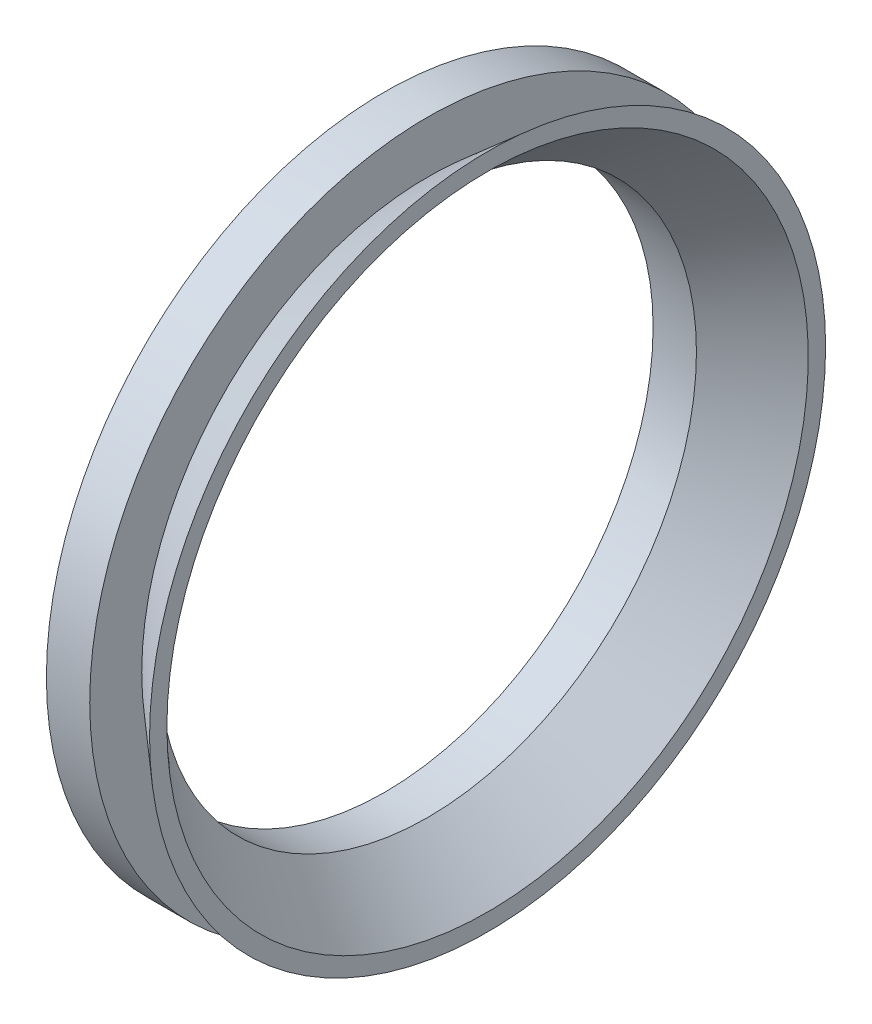
SolidWorks part; units mm, degrees
ref_plane "前视基准面" through (0, 0, 0) normal (0, 0, 1) x (1, 0, 0)
ref_plane "上视基准面" through (0, 0, 0) normal (0, 1, 0) x (1, 0, 0)
ref_plane "右视基准面" through (0, 0, 0) normal (1, 0, 0) x (0, 0, -1)
sketch "草图1" plane through (0, 0, 0) normal (0, 0, 1) x (1, 0, 0)
  line L0 (0, 0) -> (2.5, 0)
  line L1 (2.5, 0) -> (5.9511, 3)
  line L2 (0, 0) -> (0, 4)
  line L3 (0, 4) -> (2.5, 4)
  line L4 (2.5, 4) -> (2.5, 1)
  line L5 (2.5, 1) -> (5.9511, 4)
  line L6 (2.5, 4) -> (6.9465, 4) construction
  line L7 (5.9511, 4) -> (5.9511, 3)
  line L9 (-6.8703, -15.5) -> (11.3746, -15.5) construction
  dimension "D1" = 2.5
  dimension "D2" = 139
  dimension "D3" = 4
  dimension "D4" = 3
  dimension "D5" = 139
  dimension "D6" = 15.5
revolve "旋转1" add sketch "草图1" angle 360 about L9
